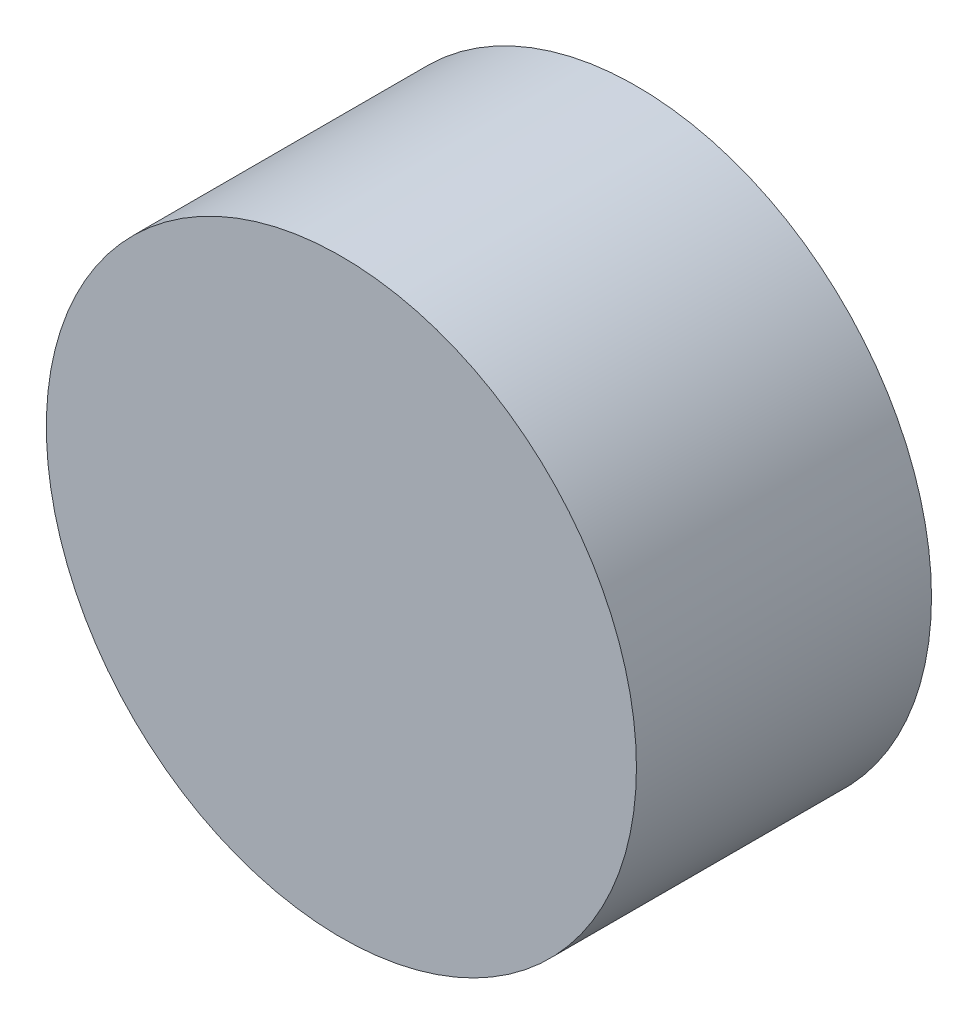
from build123d import *

# Parameters (mm, degrees)
SKETCH1_R           = 15
BOSS_EXTRUDE1_DEPTH = 15


with BuildPart() as part:
    # Sketch1 → Boss-Extrude1 (new body)
    with BuildSketch(Plane.XY):
        with Locations((52.708583994, 73.328205372)):
            Circle(SKETCH1_R)
    extrude(amount=BOSS_EXTRUDE1_DEPTH)


solid = part.part
